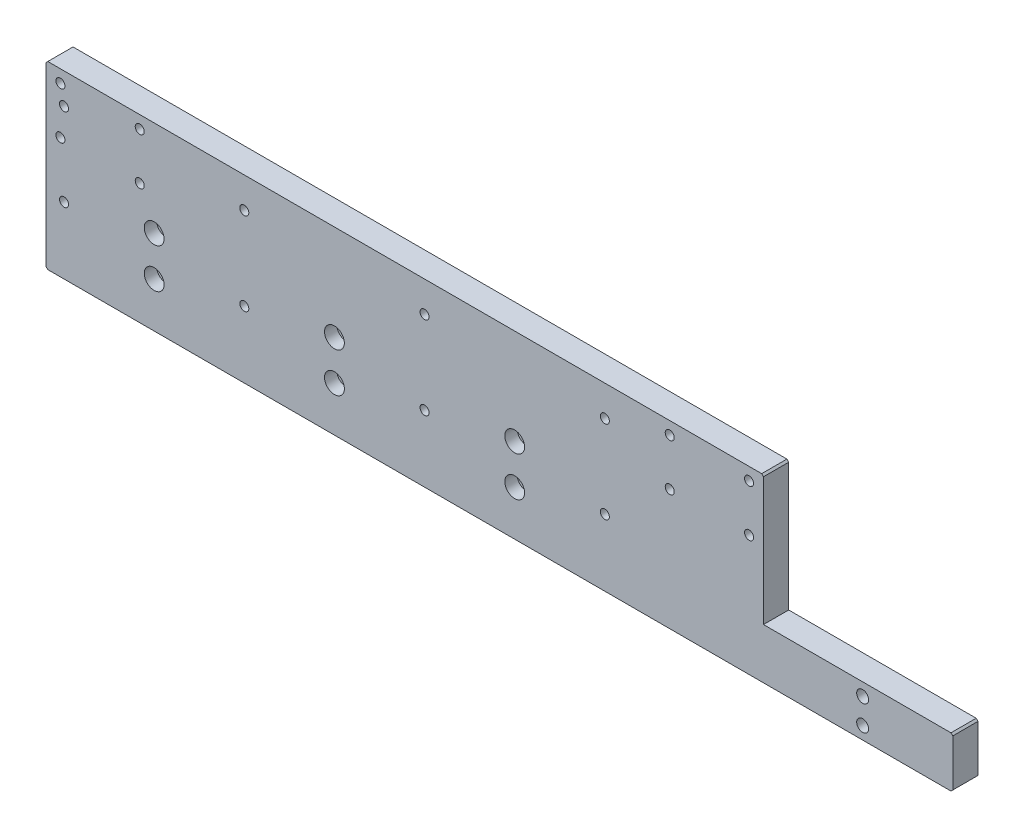
from build123d import *

# Parameters (mm, degrees)
SKETCH1_W                                            = 398
SKETCH1_H                                            = 100
BOSS_EXTRUDE1_DEPTH                                  = 7
SKETCH2_W                                            = 14
SKETCH2_H                                            = 28
BOSS_EXTRUDE2_DEPTH                                  = 105
M6_CLEARANCE_HOLE1_D                                 = 6.6
M6_TAPPED_HOLE1_D                                    = 5
HOLE_SIZE_PER_SOCKET_HEAD_CAP_SCREW_TYPE_D           = 6.6
HOLE_SIZE_PER_SOCKET_HEAD_CAP_SCREW_TYPE_CBORE_D     = 11
HOLE_SIZE_PER_SOCKET_HEAD_CAP_SCREW_TYPE_CBORE_DEPTH = 6.8
M6_TAPPED_HOLE2_D                                    = 5
M6_TAPPED_HOLE3_D                                    = 5
M6_TAPPED_HOLE3_DEPTH                                = 15
M6_TAPPED_HOLE3_TIP                                  = 1.502151548
CHAMFER1_SIZE                                        = 1


with BuildPart() as part:
    # Sketch1 → Boss-Extrude1 (new, symmetric)
    with BuildSketch(Plane.XY):
        Rectangle(SKETCH1_W, SKETCH1_H)
    extrude(amount=BOSS_EXTRUDE1_DEPTH, both=True)

    # Sketch2 → Boss-Extrude2 (add)
    with BuildSketch(Plane(origin=(199, 0, 0), x_dir=(0, 0, -1), z_dir=(1, 0, 0))):
        with Locations((0, -36)):
            Rectangle(SKETCH2_W, SKETCH2_H)
    extrude(amount=BOSS_EXTRUDE2_DEPTH)

    # M6 Clearance Hole1 (through all)
    with Locations(Plane(origin=(0, 0, -7), x_dir=(-1, 0, 0), z_dir=(0, 0, -1))):
        with Locations((-254, -43), (-254, -29)):
            Hole(M6_CLEARANCE_HOLE1_D / 2)

    # M6 Tapped Hole1 (through all)
    with Locations(Plane.XY.offset(7)):
        with Locations((111, -13), (-189, 33), (-189, -13), (-89, 33), (-89, -13), (11, 33), (11, -13), (111, 33)):
            Hole(M6_TAPPED_HOLE1_D / 2)

    # Hole Size per Socket Head Cap Screw Type1 (through all)
    with Locations(Plane.XY.offset(7)):
        with Locations((-139, -3), (61, -25), (61, -3), (-39, -25), (-39, -3), (-139, -25)):
            CounterBoreHole(HOLE_SIZE_PER_SOCKET_HEAD_CAP_SCREW_TYPE_D / 2, HOLE_SIZE_PER_SOCKET_HEAD_CAP_SCREW_TYPE_CBORE_D / 2, HOLE_SIZE_PER_SOCKET_HEAD_CAP_SCREW_TYPE_CBORE_DEPTH)

    # M6 Tapped Hole2 (through all)
    with Locations(Plane(origin=(0, 0, -7), x_dir=(-1, 0, 0), z_dir=(0, 0, -1))):
        with Locations((-191, 43), (-147, 17), (-191, 17), (-147, 43), (147, 43), (191, 17), (147, 17), (191, 43)):
            Hole(M6_TAPPED_HOLE2_D / 2)

    # M6 Tapped Hole3
    with Locations(Plane(origin=(0, -50, 0), x_dir=(-1, 0, 0), z_dir=(0, -1, 0))):
        with Locations((-291, 0), (189, 0), (89, 0), (-11, 0), (-111, 0), (-211, 0)):
            Hole(M6_TAPPED_HOLE3_D / 2, depth=M6_TAPPED_HOLE3_DEPTH)
            with Locations((0, 0, -(M6_TAPPED_HOLE3_DEPTH + M6_TAPPED_HOLE3_TIP / 2))):  # 118° drill point
                Cone(0, M6_TAPPED_HOLE3_D / 2, M6_TAPPED_HOLE3_TIP, mode=Mode.SUBTRACT)

    # Chamfer1
    chamfer1_edges = [part.edges().sort_by_distance(p)[0] for p in [
        (304, -50, 0),
        (304, -22, 0),
        (-199, -50, 0),
        (-199, 50, 0),
        (199, 50, 0),
    ]]
    chamfer(chamfer1_edges, length=CHAMFER1_SIZE)


solid = part.part
